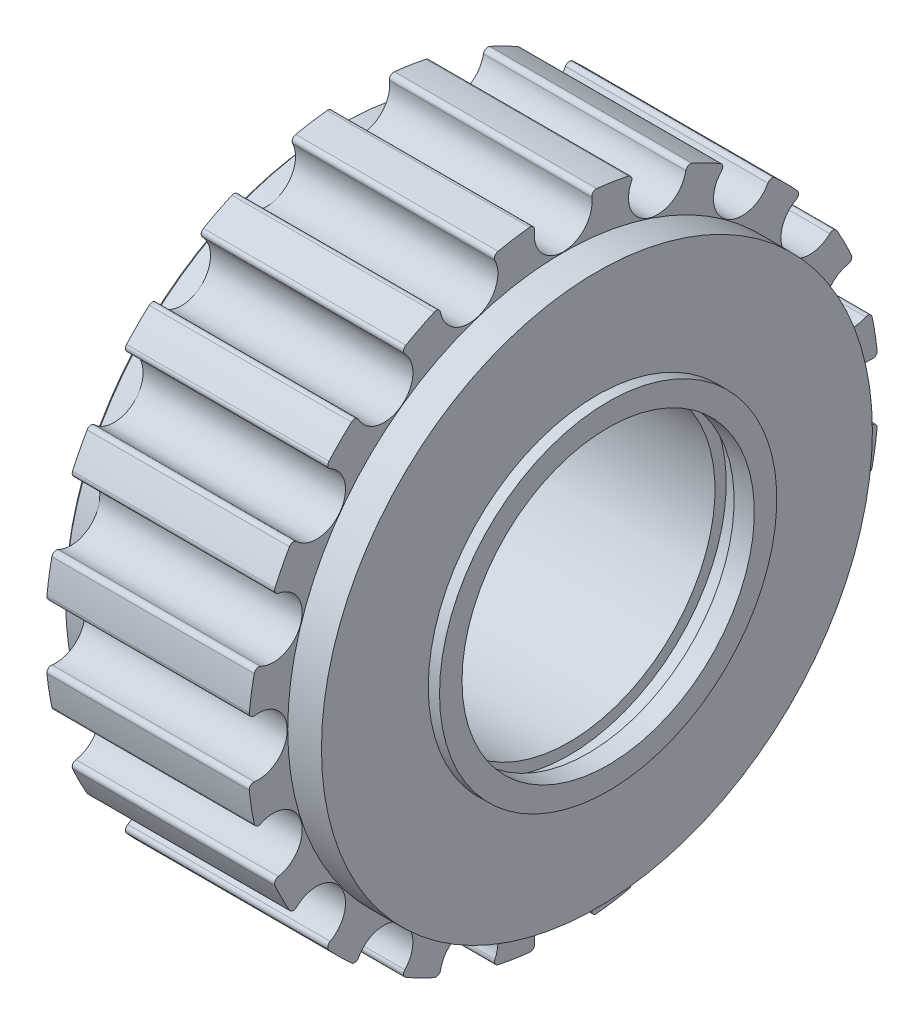
from build123d import *

# Parameters (mm, degrees)
CHAMFER_1_SIZE           = 0.25
CUT_EXTRUDE_START        = -18
CUT_EXTRUDE_1_DEPTH      = 18
PATTERN_CIRCULAR_1_COUNT = 20


with BuildPart() as part:
    # 草图1 → 旋转2 (revolve)
    with BuildSketch(Plane.XY, mode=Mode.PRIVATE) as revolve_2_sk:
        Polygon((0, 10.5), (4.5, 10.5), (4.5, 13), (20.5, 13), (20.5, 14), (22.2, 14), (22.2, 13), (24, 13), (24, 15), (23, 15), (23, 24.5), (20, 24.5), (20, 28.08), (2, 28.08), (2, 24.5), (0, 24.5), align=None)
    revolve(revolve_2_sk.sketch.rotate(Axis((0, 0, 0), (1, 0, 0)), 90), axis=Axis((0, 0, 0), (1, 0, 0)))

    # 倒角1
    chamfer_1_edges = [part.edges().sort_by_distance(p)[0] for p in [
        (0, 0, -24.5),
    ]]
    chamfer(chamfer_1_edges, length=CHAMFER_1_SIZE)

    # 草图2 → 切除-拉伸1 (cut)
    with BuildSketch(Plane(origin=(20, 0, 0), x_dir=(0, 0, -1), z_dir=(1, 0, 0)).offset(CUT_EXTRUDE_START)):
        with BuildLine():
            ThreePointArc((2.983603122, 27.921040676), (0, 28.08), (-2.983603122, 27.921040676))
            ThreePointArc((-2.983603122, 27.921040676), (-2.653608716, 27.801419798), (-2.544993686, 27.467641073))
            ThreePointArc((-2.544993686, 27.467641073), (0, 24.54), (2.544993686, 27.467641073))
            ThreePointArc((2.544993686, 27.467641073), (2.653608716, 27.801419798), (2.983603122, 27.921040676))
        make_face()
    cut_extrude_1 = extrude(amount=CUT_EXTRUDE_1_DEPTH, mode=Mode.SUBTRACT)

    # 阵列(圆周)1: 切除-拉伸1 ×20 about axis
    pattern_circular_1_axis = Axis((0, 0, 0), (1, 0, 0))
    for i in range(1, PATTERN_CIRCULAR_1_COUNT):
        add(cut_extrude_1.rotate(pattern_circular_1_axis, i * 360 / PATTERN_CIRCULAR_1_COUNT), mode=Mode.SUBTRACT)


solid = part.part
